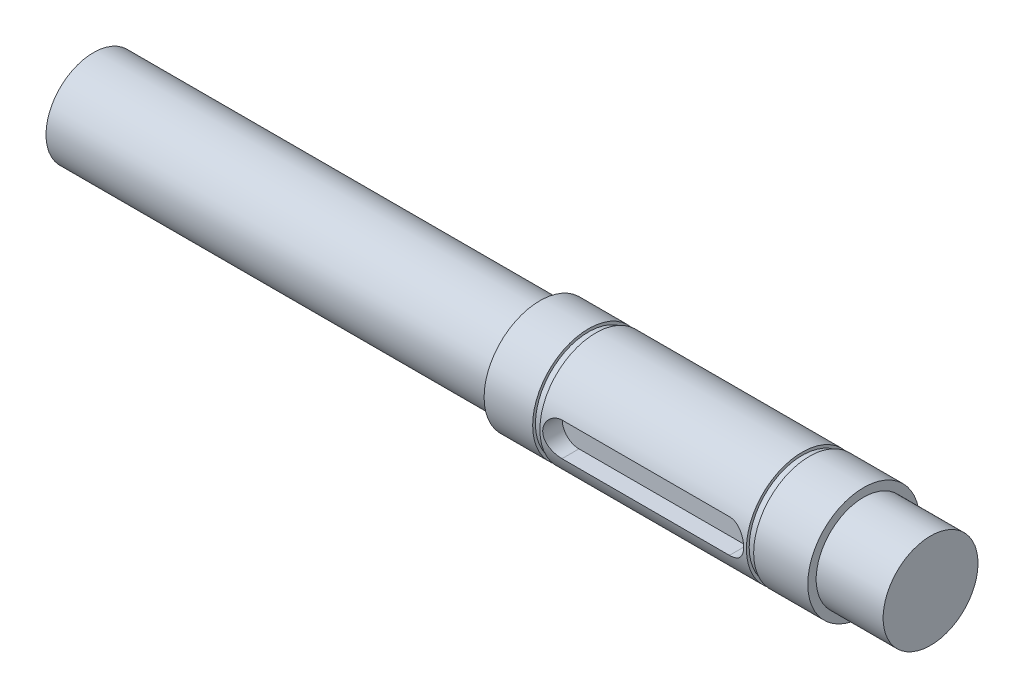
SolidWorks part; units mm, degrees
ref_plane "前视基准面" through (0, 0, 0) normal (0, 0, 1) x (1, 0, 0)
ref_plane "上视基准面" through (0, 0, 0) normal (0, 1, 0) x (1, 0, 0)
ref_plane "右视基准面" through (0, 0, 0) normal (1, 0, 0) x (0, 0, -1)
sketch "草图1" plane through (0, 0, 0) normal (1, 0, 0) x (0, 0, -1)
  circle A0 centre (0, 0) radius 10
  dimension "D1" = 20
extrude "凸台-拉伸1" add sketch "草图1" along normal blind 58
sketch "草图2" plane through (58, 0, 0) normal (1, 0, 0) x (0, 0, -1)
  circle A0 centre (0, 0) radius 8.5
  dimension "D1" = 17
extrude "凸台-拉伸2" add sketch "草图2" along normal blind 12
sketch "草图3" plane through (0, 0, 0) normal (-1, 0, 0) x (0, 0, 1)
  circle A0 centre (0, 0) radius 8.5
  dimension "D1" = 17
extrude "凸台-拉伸3" add sketch "草图3" along normal blind 80
ref_plane "基准面1" through (0, 0, 6.5) normal (0, 0, 1) x (1, 0, 0)
sketch "草图4" plane through (0, 0, 6.5) normal (0, 0, 1) x (1, 0, 0)
  line L0 (13.5, 0) -> (43.5, 0) construction
  line L1 (13.5, 3) -> (43.5, 3)
  line L2 (13.5, -3) -> (43.5, -3)
  line L3 (0, 10) -> (0, -10) construction
  arc A0 (13.5, 3) -> (13.5, -3) centre (13.5, 0) ccw
  arc A1 (43.5, -3) -> (43.5, 3) centre (43.5, 0) ccw
  point P3 (28.5, 0)
  dimension "D1" = 6
  dimension "D2" = 30
  dimension "D3" = 28.5
extrude "切除-拉伸1" cut sketch "草图4" along normal through all
sketch "草图5" plane through (0, 0, 0) normal (0, 1, 0) x (1, 0, 0)
  line L0 (0, 0) -> (29.4242, 0) construction
  line L1 (58, 10) -> (0, 10) construction
  line L2 (8.7, 10) -> (10, 10)
  line L3 (8.7, 10) -> (8.7, 9.5)
  line L4 (8.7, 9.5) -> (10, 9.5)
  line L5 (10, 10) -> (10, 9.5)
  line L7 (47, 10) -> (48.3, 10)
  line L8 (47, 10) -> (47, 9.5)
  line L9 (47, 9.5) -> (48.3, 9.5)
  line L10 (48.3, 10) -> (48.3, 9.5)
  line L11 (0, 10) -> (0, -10) construction
  dimension "D1" = 1.3
  dimension "D2" = 9.5
  dimension "D3" = 10
  dimension "D4" = 37
revolve "切除-旋转1" cut sketch "草图5" angle 360 about L0
